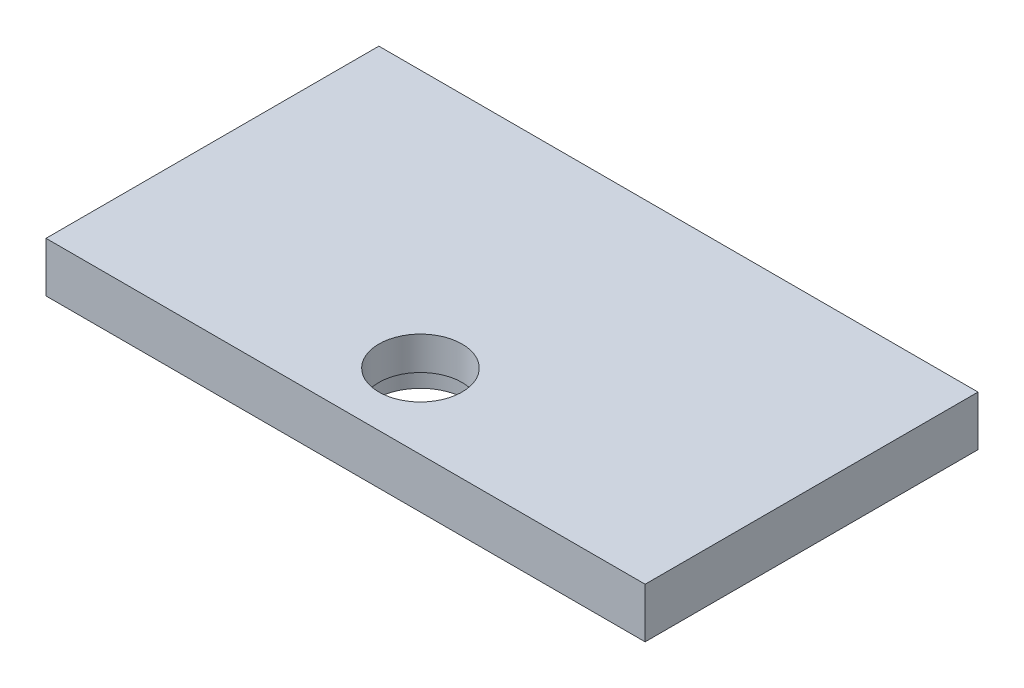
SolidWorks part; units mm, degrees
ref_plane "前视基准面" through (0, 0, 0) normal (0, 0, 1) x (1, 0, 0)
ref_plane "上视基准面" through (0, 0, 0) normal (0, 1, 0) x (1, 0, 0)
ref_plane "右视基准面" through (0, 0, 0) normal (1, 0, 0) x (0, 0, -1)
sketch "草图1" plane through (0, 0, 0) normal (0, 1, 0) x (1, 0, 0)
  line L1 (-180, -100) -> (180, -100)
  line L2 (-180, -100) -> (-180, 100)
  line L3 (-180, 100) -> (180, 100)
  line L4 (180, -100) -> (180, 100)
  line L5 (-180, -100) -> (180, 100) construction
  line L6 (-180, 100) -> (180, -100) construction
  point P0 (0, 0)
  dimension "D1" = 200
  dimension "D2" = 360
extrude "凸台-拉伸1" add sketch "草图1" along normal blind 30
sketch "草图2" plane through (0, 0, 0) normal (0, -1, 0) x (1, 0, 0)
  line L6 (-180, 100) -> (180, 100) construction
  circle A0 centre (0, 55) radius 25
  dimension "D1" = 50
  dimension "D2" = 20
extrude "切除-拉伸1" cut sketch "草图2" against normal through all
sketch "草图3" plane through (0, 0, 0) normal (0, -1, 0) x (1, 0, 0)
  line L5 (-180, 100) -> (180, 100) construction
  circle A0 centre (0, 55) radius 27.5
  dimension "D1" = 17.5
  dimension "D2" = 55
extrude "切除-拉伸2" cut sketch "草图3" against normal blind 10
